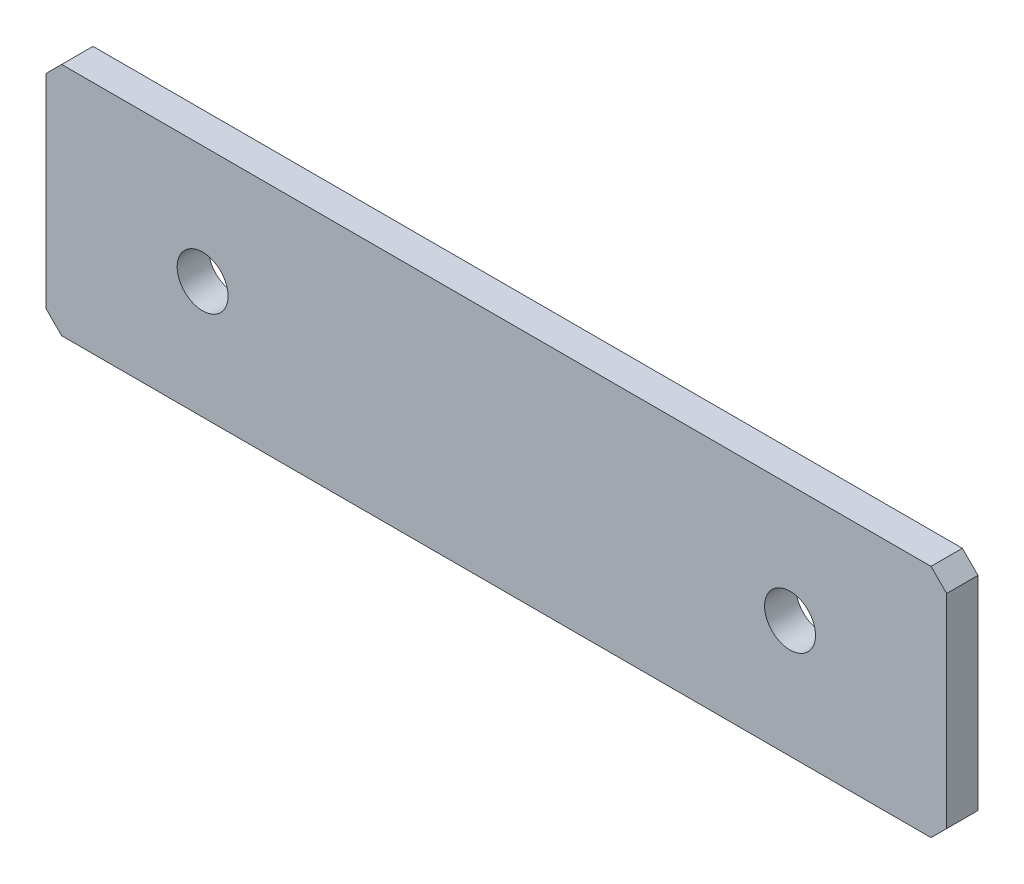
from build123d import *

# Parameters (mm, degrees)
SKETCH1_W           = 115
SKETCH1_H           = 30
SKETCH1_R           = 3.25
BOSS_EXTRUDE1_DEPTH = 4
CHAMFER1_SIZE       = 2


with BuildPart() as part:
    # Sketch1 → Boss-Extrude1 (new body)
    with BuildSketch(Plane.XY):
        Rectangle(SKETCH1_W, SKETCH1_H)
        with Locations((-37.5, 0)):
            Circle(SKETCH1_R, mode=Mode.SUBTRACT)
        with Locations((37.5, 0)):
            Circle(SKETCH1_R, mode=Mode.SUBTRACT)
    extrude(amount=BOSS_EXTRUDE1_DEPTH)

    # Chamfer1
    chamfer1_edges = [part.edges().sort_by_distance(p)[0] for p in [
        (-57.5, 15, 2),
        (57.5, 15, 2),
        (57.5, -15, 2),
        (-57.5, -15, 2),
    ]]
    chamfer(chamfer1_edges, length=CHAMFER1_SIZE)


solid = part.part
